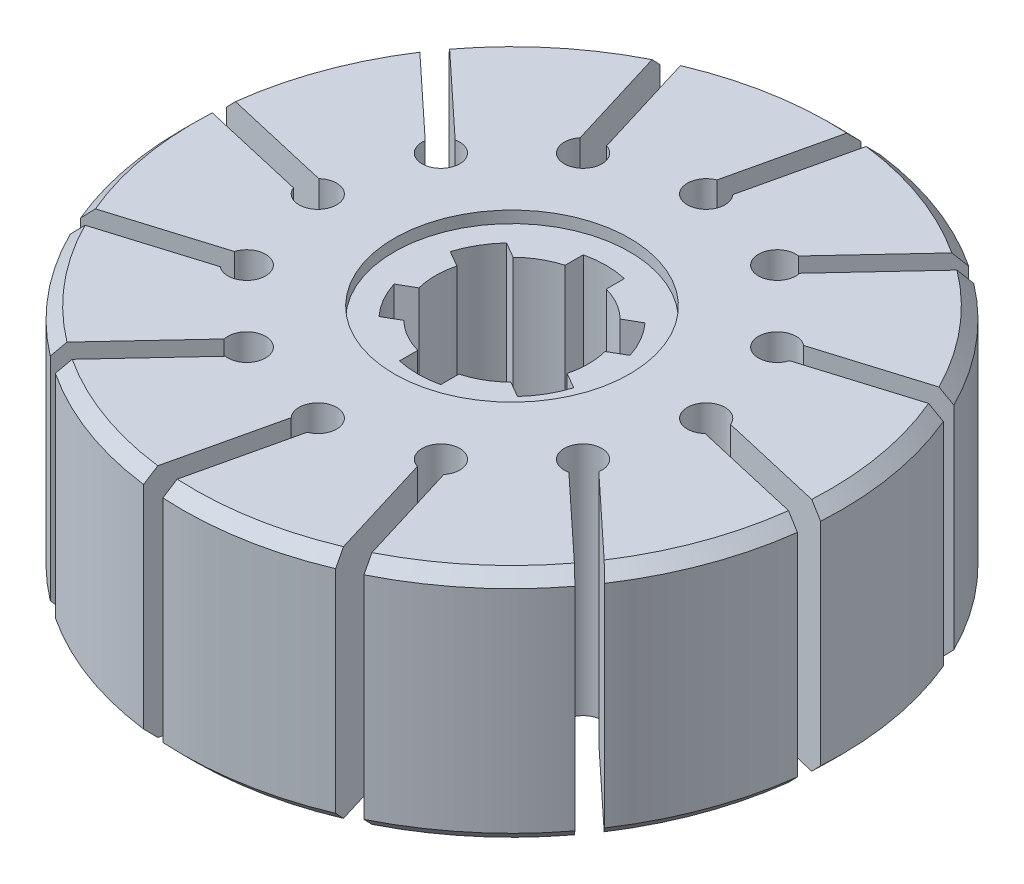
SolidWorks part; units mm, degrees
ref_plane "Front Plane" through (0, 0, 0) normal (0, 0, 1) x (1, 0, 0)
ref_plane "Top Plane" through (0, 0, 0) normal (0, 1, 0) x (1, 0, 0)
ref_plane "Right Plane" through (0, 0, 0) normal (1, 0, 0) x (0, 0, -1)
other "Configuration Table"
sketch "Sketch1" plane through (0, 0, 0) normal (0, 1, 0) x (1, 0, 0)
  circle A0 centre (0, 0) radius 28
  dimension "D1" = 56
extrude "Boss-Extrude1" add sketch "Sketch1" along normal blind 20
sketch "Sketch2" plane through (0, 20, 0) normal (0, 1, 0) x (1, 0, 0)
  circle A0 centre (0, 0) radius 10
  dimension "D1" = 20
extrude "Cut-Extrude1" cut sketch "Sketch2" against normal blind 1
sketch "Sketch3" plane through (0, 19, 0) normal (0, 1, 0) x (1, 0, 0)
  line L0 (0, 0) -> (0, 12.5157) construction
  line L1 (-1.75, 7.8062) -> (-1.75, 6.26)
  line L2 (1.75, 7.8062) -> (1.75, 6.26)
  line L3 (5.8854, 5.4187) -> (4.5463, 4.6455)
  line L4 (7.6354, 2.3876) -> (6.2963, 1.6145)
  line L5 (7.6354, -2.3876) -> (6.2963, -1.6145)
  line L6 (5.8854, -5.4187) -> (4.5463, -4.6455)
  line L7 (1.75, -7.8062) -> (1.75, -6.26)
  line L8 (-1.75, -7.8062) -> (-1.75, -6.26)
  line L9 (-5.8854, -5.4187) -> (-4.5463, -4.6455)
  line L10 (-7.6354, -2.3876) -> (-6.2963, -1.6145)
  line L11 (-7.6354, 2.3876) -> (-6.2963, 1.6145)
  line L12 (-5.8854, 5.4187) -> (-4.5463, 4.6455)
  arc A0 (1.75, 7.8062) -> (-1.75, 7.8062) centre (0, 0) ccw
  arc A1 (4.5463, 4.6455) -> (1.75, 6.26) centre (0, 0) ccw
  arc A2 (7.6354, 2.3876) -> (5.8854, 5.4187) centre (0, 0) ccw
  arc A3 (5.8854, -5.4187) -> (7.6354, -2.3876) centre (0, 0) ccw
  arc A4 (-1.75, -7.8062) -> (1.75, -7.8062) centre (0, 0) ccw
  arc A5 (-7.6354, -2.3876) -> (-5.8854, -5.4187) centre (0, 0) ccw
  arc A6 (-5.8854, 5.4187) -> (-7.6354, 2.3876) centre (0, 0) ccw
  arc A7 (-1.75, 6.26) -> (-4.5463, 4.6455) centre (0, 0) ccw
  arc A8 (6.2963, -1.6145) -> (6.2963, 1.6145) centre (0, 0) ccw
  arc A9 (1.75, -6.26) -> (4.5463, -4.6455) centre (0, 0) ccw
  arc A10 (-4.5463, -4.6455) -> (-1.75, -6.26) centre (0, 0) ccw
  arc A11 (-6.2963, 1.6145) -> (-6.2963, -1.6145) centre (0, 0) ccw
  point P30 (0, 0)
  dimension "D1" = 16
  dimension "D2" = 13
  dimension "D3" = 3.5
  dimension "D4" = 6
extrude "Cut-Extrude2" cut sketch "Sketch3" against normal blind 30
sketch "Sketch4" plane through (0, 0, 0) normal (0, -1, 0) x (-1, 0, 0)
  circle A0 centre (0, 0) radius 10
  dimension "D1" = 20
extrude "Cut-Extrude3" cut sketch "Sketch4" against normal blind 1
sketch "Sketch5" plane through (0, 20, 0) normal (0, 1, 0) x (1, 0, 0)
  circle A0 centre (0, 0) radius 16.5 construction
  circle A1 centre (0, 16.5) radius 1.6
  circle A2 centre (8.25, 14.2894) radius 1.6
  circle A3 centre (14.2894, 8.25) radius 1.6
  circle A4 centre (16.5, 0) radius 1.6
  circle A5 centre (14.2894, -8.25) radius 1.6
  circle A6 centre (8.25, -14.2894) radius 1.6
  circle A7 centre (0, -16.5) radius 1.6
  circle A8 centre (-8.25, -14.2894) radius 1.6
  circle A9 centre (-14.2894, -8.25) radius 1.6
  circle A10 centre (-16.5, 0) radius 1.6
  circle A11 centre (-14.2894, 8.25) radius 1.6
  circle A12 centre (-8.25, 14.2894) radius 1.6
  point P30 (0, 0)
  dimension "D1" = 33
  dimension "D2" = 3.2
  dimension "D3" = 12
extrude "Cut-Extrude4" cut sketch "Sketch5" against normal blind 80
chamfer "Chamfer1" distance 1 angle 45 2 edges at (0, 0, 28) (0, 20, 28)
sketch "Sketch6" plane through (0, 20, 0) normal (0, 1, 0) x (1, 0, 0)
  line L0 (0, 0) -> (0, 33.367) construction
  line L1 (0, 16.5) -> (3.3185, 30.8742) construction
  line L2 (0.8769, 16.2975) -> (4.1955, 30.6717)
  line L3 (-0.8769, 16.7025) -> (2.4416, 31.0766)
  line L4 (2.4416, 31.0766) -> (4.1955, 30.6717)
  line L5 (-0.8769, 16.7025) -> (0.8769, 16.2975)
  line L6 (7.5918, 14.9032) -> (8.9082, 13.6756)
  line L7 (8.9082, 13.6756) -> (18.9692, 24.4648)
  line L8 (17.6528, 25.6923) -> (18.9692, 24.4648)
  line L9 (7.5918, 14.9032) -> (17.6528, 25.6923)
  line L10 (14.0263, 9.1107) -> (14.5526, 7.3893)
  line L11 (14.5526, 7.3893) -> (28.6602, 11.7025)
  line L12 (28.134, 13.4238) -> (28.6602, 11.7025)
  line L13 (14.0263, 9.1107) -> (28.134, 13.4238)
  line L14 (16.7025, 0.8769) -> (16.2975, -0.8769)
  line L15 (16.2975, -0.8769) -> (30.6717, -4.1955)
  line L16 (31.0766, -2.4416) -> (30.6717, -4.1955)
  line L17 (16.7025, 0.8769) -> (31.0766, -2.4416)
  line L18 (14.9032, -7.5918) -> (13.6756, -8.9082)
  line L19 (13.6756, -8.9082) -> (24.4648, -18.9692)
  line L20 (25.6923, -17.6528) -> (24.4648, -18.9692)
  line L21 (14.9032, -7.5918) -> (25.6923, -17.6528)
  line L22 (9.1107, -14.0263) -> (7.3893, -14.5526)
  line L23 (7.3893, -14.5526) -> (11.7025, -28.6602)
  line L24 (13.4238, -28.134) -> (11.7025, -28.6602)
  line L25 (9.1107, -14.0263) -> (13.4238, -28.134)
  line L26 (0.8769, -16.7025) -> (-0.8769, -16.2975)
  line L27 (-0.8769, -16.2975) -> (-4.1955, -30.6717)
  line L28 (-2.4416, -31.0766) -> (-4.1955, -30.6717)
  line L29 (0.8769, -16.7025) -> (-2.4416, -31.0766)
  line L30 (-7.5918, -14.9032) -> (-8.9082, -13.6756)
  line L31 (-8.9082, -13.6756) -> (-18.9692, -24.4648)
  line L32 (-17.6528, -25.6923) -> (-18.9692, -24.4648)
  line L33 (-7.5918, -14.9032) -> (-17.6528, -25.6923)
  line L34 (-14.0263, -9.1107) -> (-14.5526, -7.3893)
  line L35 (-14.5526, -7.3893) -> (-28.6602, -11.7025)
  line L36 (-28.134, -13.4238) -> (-28.6602, -11.7025)
  line L37 (-14.0263, -9.1107) -> (-28.134, -13.4238)
  line L38 (-16.7025, -0.8769) -> (-16.2975, 0.8769)
  line L39 (-16.2975, 0.8769) -> (-30.6717, 4.1955)
  line L40 (-31.0766, 2.4416) -> (-30.6717, 4.1955)
  line L41 (-16.7025, -0.8769) -> (-31.0766, 2.4416)
  line L42 (-14.9032, 7.5918) -> (-13.6756, 8.9082)
  line L43 (-13.6756, 8.9082) -> (-24.4648, 18.9692)
  line L44 (-25.6923, 17.6528) -> (-24.4648, 18.9692)
  line L45 (-14.9032, 7.5918) -> (-25.6923, 17.6528)
  line L46 (-9.1107, 14.0263) -> (-7.3893, 14.5526)
  line L47 (-7.3893, 14.5526) -> (-11.7025, 28.6602)
  line L48 (-13.4238, 28.134) -> (-11.7025, 28.6602)
  line L49 (-9.1107, 14.0263) -> (-13.4238, 28.134)
  point P56 (0, 0)
  dimension "D1" = 13
  dimension "D4" = 12
  dimension "D2" = 0.9
  dimension "D3" = 0.9
extrude "Cut-Extrude5" cut sketch "Sketch6" against normal blind 80
